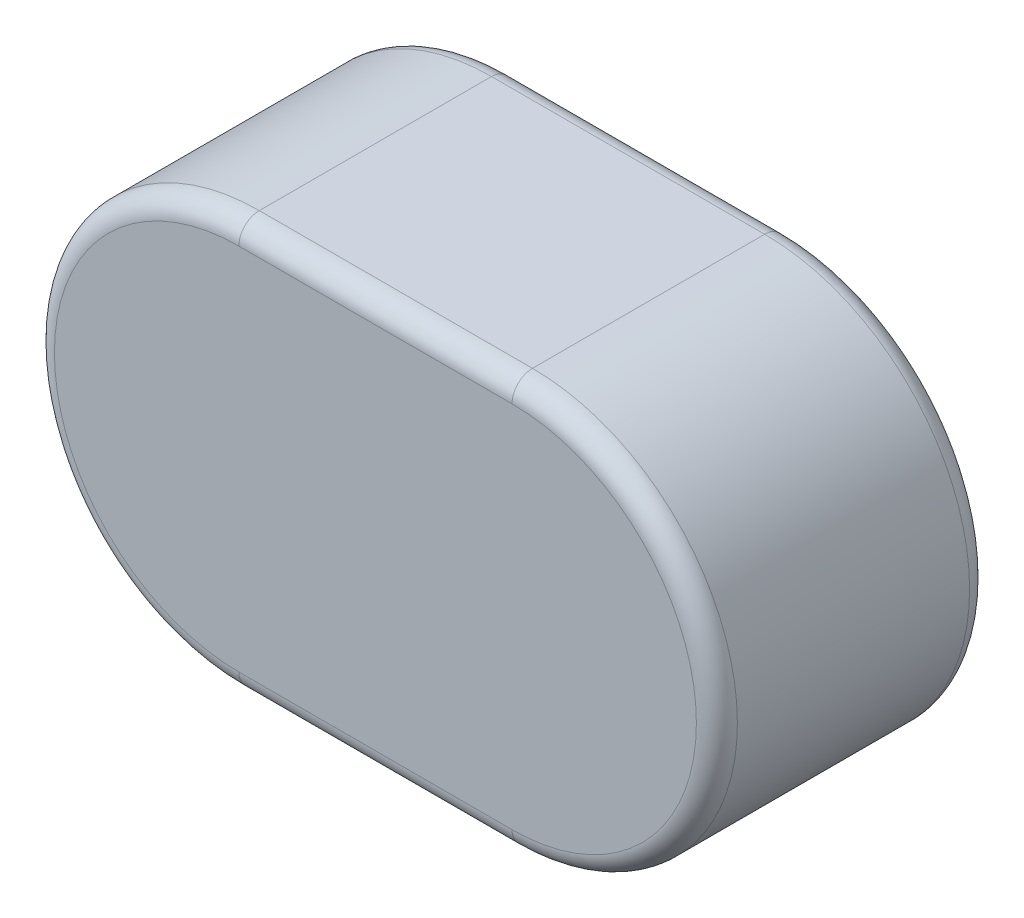
SolidWorks part; units mm, degrees
material "45"
ref_plane "基准面1" through (0, 0, 0) normal (0, 0, 1) x (1, 0, 0)
ref_plane "基准面2" through (0, 0, 0) normal (0, 1, 0) x (1, 0, 0)
ref_plane "基准面3" through (0, 0, 0) normal (1, 0, 0) x (0, 0, -1)
sketch "尺寸草图" plane through (0, 0, 0) normal (0, 0, 1) x (1, 0, 0)
  line L0 (-10, 0) -> (10, 0) construction
  point P3 (-8, 0)
  point P4 (-0.6, 0)
  point P5 (0, 0)
  point P8 (-12, 0)
  point P11 (0, 0)
sketch "草图1" plane through (0, 0, 0) normal (0, 0, 1) x (1, 0, 0)
  line L0 (-28.0599, 0) -> (30.562, 0) construction
  line L1 (-4, 6) -> (4, 6)
  line L2 (-4, -6) -> (4, -6)
  line L3 (0, 2.9108) -> (0, -2.1805) construction
  arc A0 (-4, 6) -> (-4, -6) centre (-4, 0) ccw
  arc A1 (4, 6) -> (4, -6) centre (4, 0) cw
extrude "基体-拉伸" add sketch "草图1" along normal blind 8
fillet "圆角1" radius 0.6 8 edges at (10, 0, 8) (0, 6, 8) (-10, 0, 8) (0, 6, 0) (10, 0, 0) (0, -6, 0) (-10, 0, 0) (0, -6, 8)
equation "\"D3@草图1\" = \"L@尺寸草图\""
equation "\"D1@草图1\" = \"b@尺寸草图\" / 2"
equation "\"D1@圆角1\" = \"r@尺寸草图\""
equation "\"D1@基体-拉伸\" = \"h@尺寸草图\""
